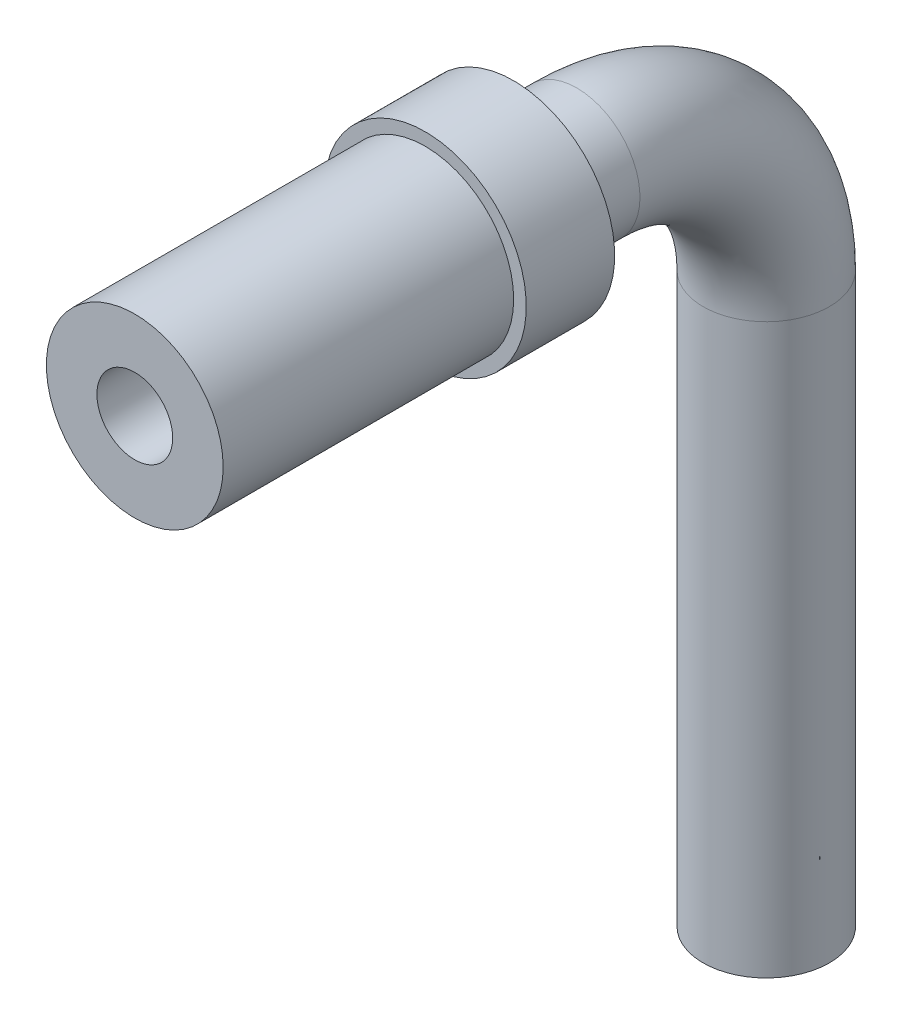
SolidWorks part; units mm, degrees
material "45#"
ref_plane "Front Plane" through (0, 0, 0) normal (0, 0, 1) x (1, 0, 0)
ref_plane "Top Plane" through (0, 0, 0) normal (0, 1, 0) x (1, 0, 0)
ref_plane "Right Plane" through (0, 0, 0) normal (1, 0, 0) x (0, 0, -1)
sketch "Sketch1" plane through (0, 0, 0) normal (1, 0, 0) x (0, 0, -1)
  line L0 (0, 0) -> (35, 0)
  line L1 (50, -15) -> (50, -60)
  arc A0 (35, 0) -> (50, -15) centre (35, -15) cw
  point P6 (50, 0)
  dimension "D3" = 15
  dimension "D1" = 50
  dimension "D2" = 60
sketch "Sketch2" plane through (0, 0, 0) normal (0, 0, 1) x (1, 0, 0)
  circle A0 centre (0, 0) radius 3
  circle A1 centre (0, 0) radius 5
  dimension "D1" = 6
  dimension "D2" = 10
sweep "Sweep1" add profiles "Sketch2" path "Sketch1"
sketch "Sketch3" plane through (0, 0, 0) normal (0, 0, 1) x (1, 0, 0)
  circle A0 centre (0, 0) radius 5
  circle A1 centre (0, 0) radius 7
  dimension "D1" = 14
  dimension "D2" = 10
extrude "Boss-Extrude1" add sketch "Sketch3" against normal blind 30
sketch "Sketch4" plane through (0, 0, -30) normal (0, 0, -1) x (-1, 0, 0)
  circle A0 centre (0, 0) radius 8
  circle A1 centre (0, 0) radius 7 construction
  circle A2 centre (0, 0) radius 7
  dimension "D1" = 16
extrude "Boss-Extrude2" add sketch "Sketch4" against normal blind 7
